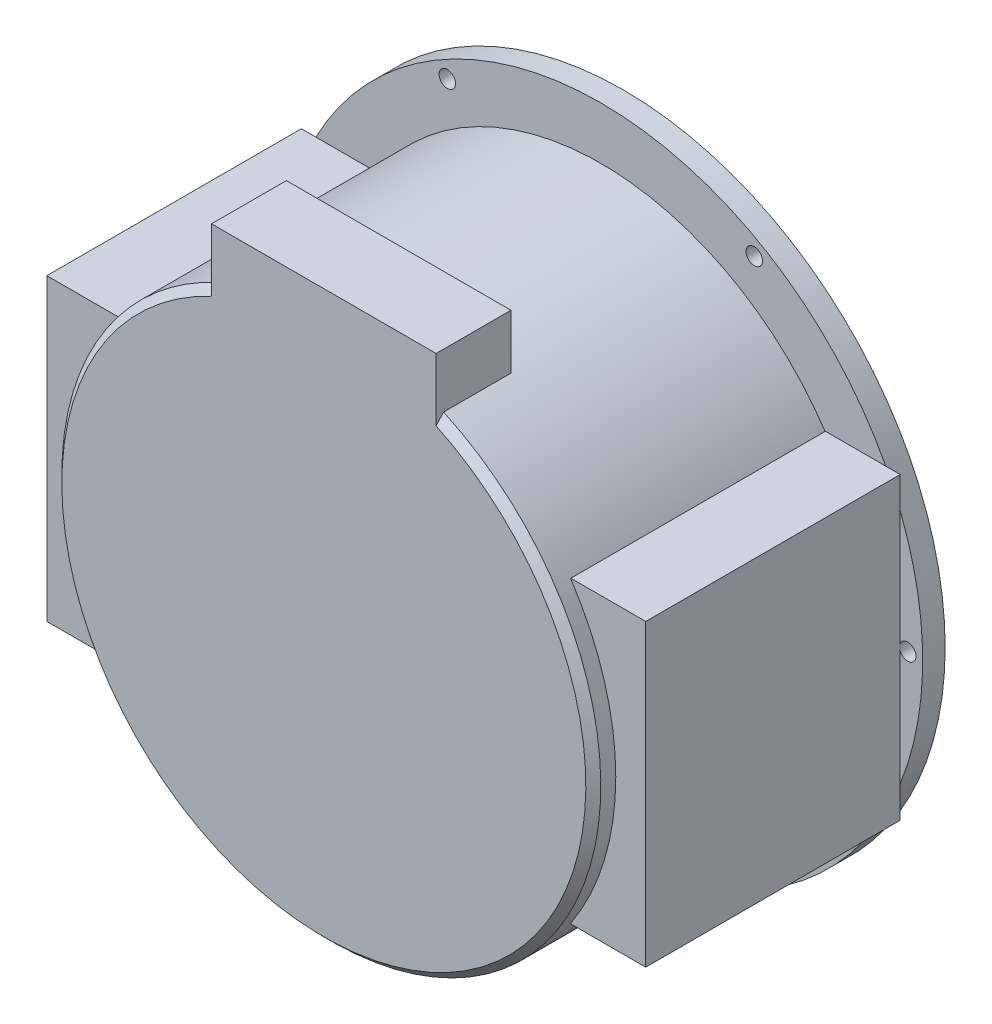
from build123d import *

# Parameters (mm, degrees)
SKETCH1_R           = 180
BOSS_EXTRUDE1_DEPTH = 100
SKETCH2_R           = 25
CUT_EXTRUDE1_DEPTH  = 80
SKETCH3_W           = 150
SKETCH3_H           = 62.418974348
BOSS_EXTRUDE3_DEPTH = 50
BOSS_EXTRUDE4_START = -15
SKETCH4_R           = 215
SKETCH4_R_2         = 180
SKETCH4_R_3         = 5.5
BOSS_EXTRUDE4_DEPTH = 15
CHAMFER1_SIZE       = 5
BOSS_EXTRUDE5_START = 150
SKETCH5_W           = 170
SKETCH5_H           = 200
BOSS_EXTRUDE5_DEPTH = 50


with BuildPart() as part:
    # Sketch1 → Boss-Extrude1 (new, symmetric)
    with BuildSketch(Plane.XY):
        Circle(SKETCH1_R)
    extrude(amount=BOSS_EXTRUDE1_DEPTH, both=True)

    # Sketch2 → Cut-Extrude1 (cut)
    with BuildSketch(Plane(origin=(0, 0, -100), x_dir=(-1, 0, 0), z_dir=(0, 0, -1))):
        Circle(SKETCH2_R)
    extrude(amount=-CUT_EXTRUDE1_DEPTH, mode=Mode.SUBTRACT)

    # Sketch3 → Boss-Extrude3 (add)
    with BuildSketch(Plane.XY.offset(100)):
        with Locations((0, 168.790512826)):
            Rectangle(SKETCH3_W, SKETCH3_H)
    extrude(amount=-BOSS_EXTRUDE3_DEPTH)

    # Sketch4 → Boss-Extrude4 (add)
    with BuildSketch(Plane(origin=(0, 0, -100), x_dir=(-1, 0, 0), z_dir=(0, 0, -1)).offset(BOSS_EXTRUDE4_START)):
        Circle(SKETCH4_R)
        Circle(SKETCH4_R_2, mode=Mode.SUBTRACT)
        with Locations((-102.5, 177.535207776)):
            Circle(SKETCH4_R_3, mode=Mode.SUBTRACT)
        with Locations((102.5, 177.535207776)):
            Circle(SKETCH4_R_3, mode=Mode.SUBTRACT)
        with Locations((205, 0)):
            Circle(SKETCH4_R_3, mode=Mode.SUBTRACT)
        with Locations((102.5, -177.535207776)):
            Circle(SKETCH4_R_3, mode=Mode.SUBTRACT)
        with Locations((-102.5, -177.535207776)):
            Circle(SKETCH4_R_3, mode=Mode.SUBTRACT)
        with Locations((-205, 0)):
            Circle(SKETCH4_R_3, mode=Mode.SUBTRACT)
    extrude(amount=BOSS_EXTRUDE4_DEPTH)

    # Chamfer1
    chamfer1_edges = [part.edges().sort_by_distance(p)[0] for p in [
        (-97.211110476, -151.492574075, 100),
    ]]
    chamfer(chamfer1_edges, length=CHAMFER1_SIZE)

    # Sketch5 → Boss-Extrude5 (add)
    with BuildSketch(Plane(origin=(0, 0, 0), x_dir=(0, 0, -1), z_dir=(1, 0, 0)).offset(BOSS_EXTRUDE5_START)):
        Rectangle(SKETCH5_W, SKETCH5_H)
    boss_extrude5 = extrude(amount=BOSS_EXTRUDE5_DEPTH)

    # Mirror1: Boss-Extrude5 across plane
    add(boss_extrude5.mirror(Plane(origin=(0, 0, 0), x_dir=(0, 0, 1), z_dir=(1, 0, 0))))


solid = part.part
